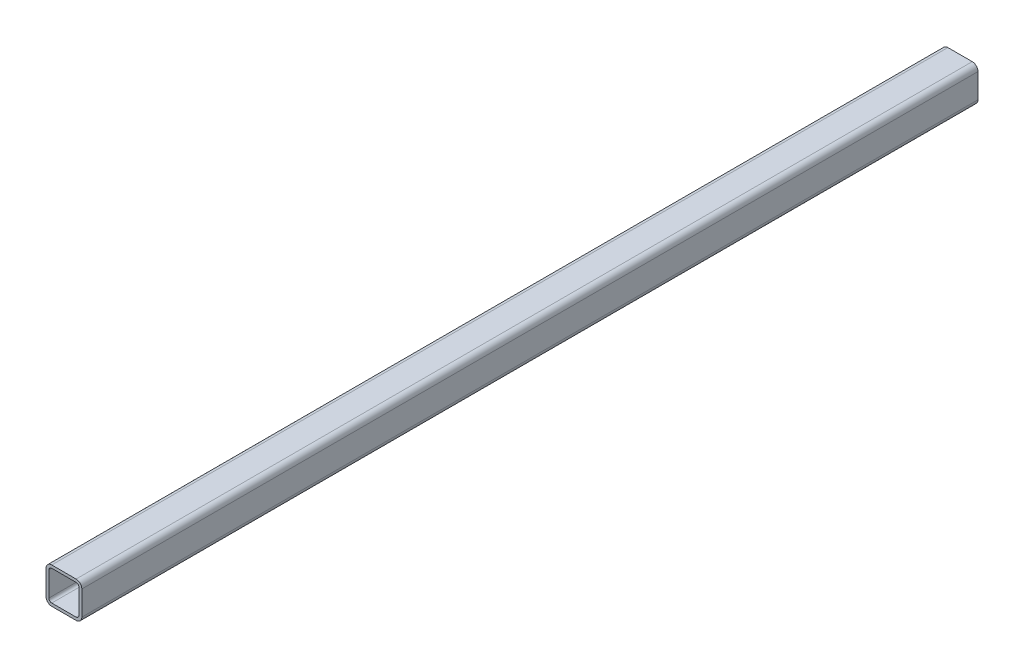
SolidWorks part; units mm, degrees
material "AISI 1045 钢，冷拔"
ref_plane "Front Plane" through (0, 0, 0) normal (0, 0, 1) x (1, 0, 0)
ref_plane "Top Plane" through (0, 0, 0) normal (0, 1, 0) x (1, 0, 0)
ref_plane "Right Plane" through (0, 0, 0) normal (1, 0, 0) x (0, 0, -1)
sketch "Sketch1" plane through (0, 0, 0) normal (0, 0, 1) x (1, 0, 0)
  line L0 (-21.0947, 0) -> (28.2454, 0) construction
  line L1 (0, 28.305) -> (0, -28.2454) construction
  line L2 (-17, 21) -> (17, 21)
  line L3 (-17, -25) -> (17, -25)
  line L4 (-25, -17) -> (-25, 17)
  line L5 (-17, 25) -> (17, 25)
  line L6 (25, -17) -> (25, 17)
  line L7 (-25, -25) -> (25, 25) construction
  line L8 (-25, 25) -> (25, -25) construction
  line L9 (21, -17) -> (21, 17)
  line L10 (-17, -21) -> (17, -21)
  line L11 (-21, -17) -> (-21, 17)
  arc A0 (17, -25) -> (25, -17) centre (17, -17) ccw
  arc A1 (-17, -25) -> (-25, -17) centre (-17, -17) cw
  arc A2 (17, 25) -> (25, 17) centre (17, 17) cw
  arc A3 (-25, 17) -> (-17, 25) centre (-17, 17) cw
  arc A4 (-21, 17) -> (-17, 21) centre (-17, 17) cw
  arc A5 (17, 21) -> (21, 17) centre (17, 17) cw
  arc A6 (17, -21) -> (21, -17) centre (17, -17) ccw
  arc A7 (-17, -21) -> (-21, -17) centre (-17, -17) cw
  point P5 (0, 0)
  dimension "D3" = 8
  dimension "D1" = 50
  dimension "D2" = 50
  dimension "D4" = 4
extrude "Boss-Extrude1" add sketch "Sketch1" along normal mid plane 1250
